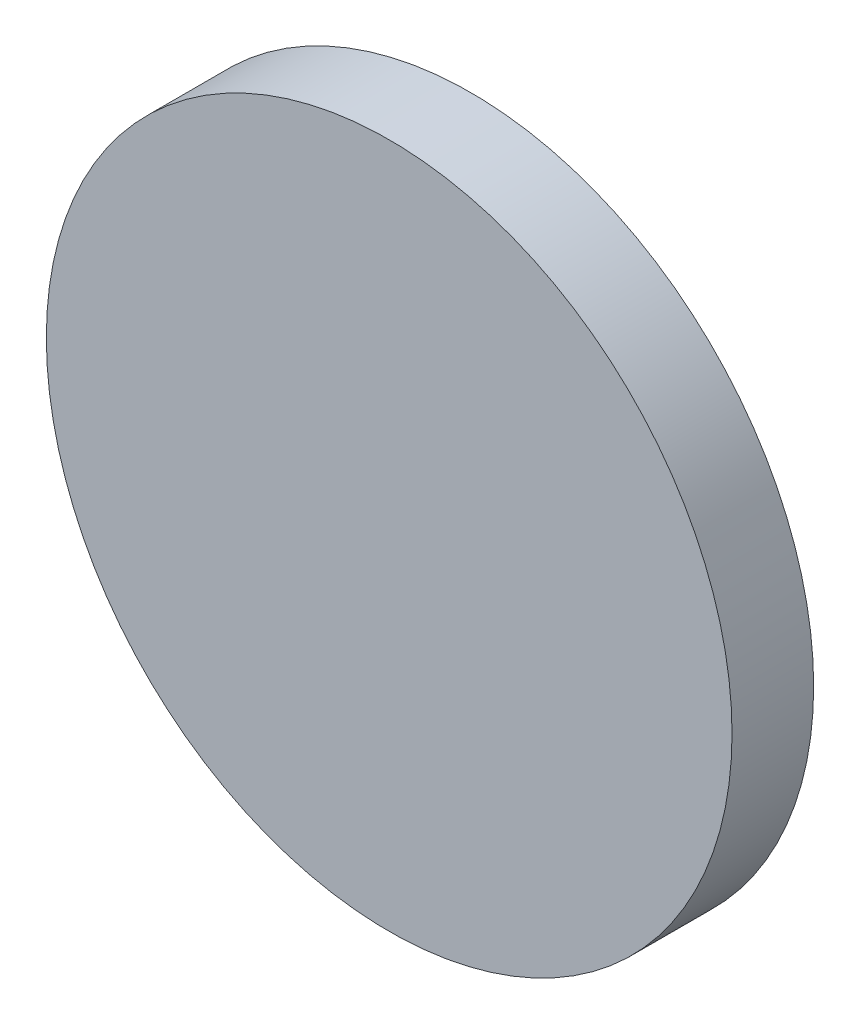
SolidWorks part; units mm, degrees
ref_plane "前视基准面" through (0, 0, 0) normal (0, 0, 1) x (1, 0, 0)
ref_plane "上视基准面" through (0, 0, 0) normal (0, 1, 0) x (1, 0, 0)
ref_plane "右视基准面" through (0, 0, 0) normal (1, 0, 0) x (0, 0, -1)
other "Configuration Table"
sketch "草图1" plane through (0, 0, 0) normal (0, 0, 1) x (1, 0, 0)
  circle A0 centre (0, 0) radius 42
  point P0 (0, 0)
  dimension "D1" = 84
extrude "凸台-拉伸1" add sketch "草图1" against normal mid plane 10
